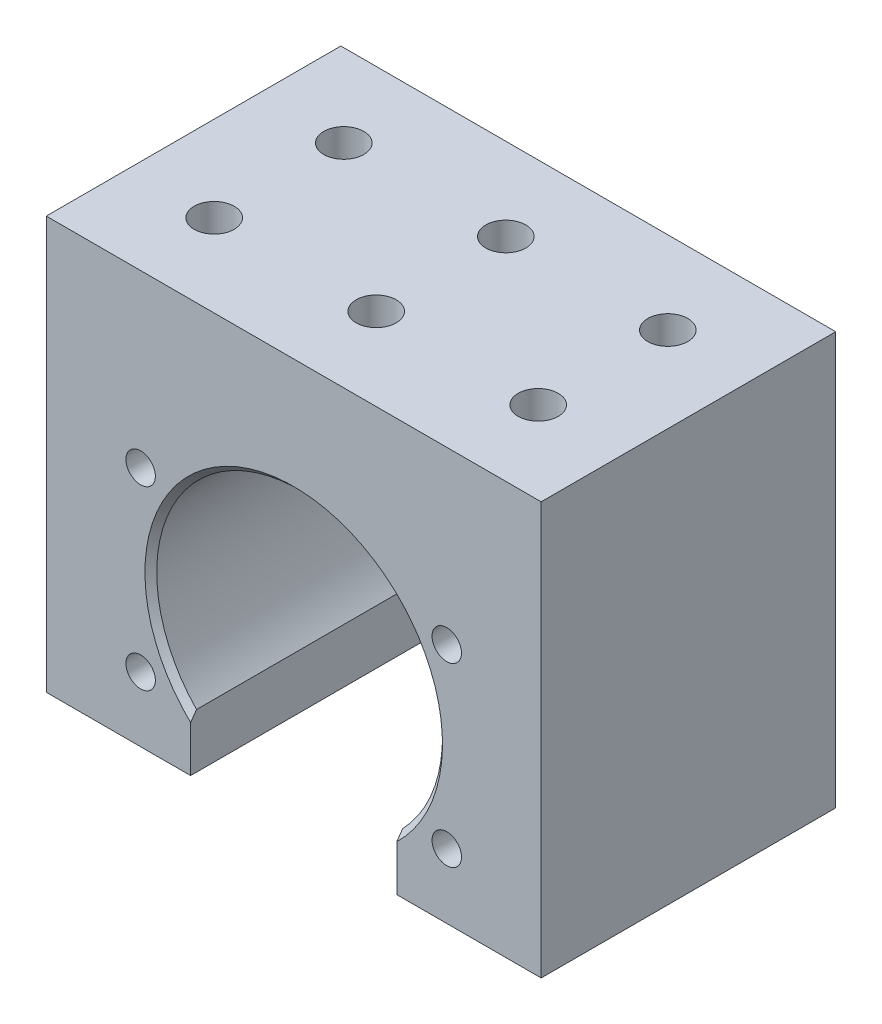
from build123d import *

# Parameters (mm, degrees)
SKETCH_1_W             = 84
SKETCH_1_H             = 70
SKETCH_1_R             = 24.25
EXTRUDE_1_DEPTH        = 25
SKETCH_2_W             = 35
SKETCH_2_H             = 9.212728036
CUT_EXTRUDE_1_DEPTH    = 75.087785768
HOLE_WIZARD_M6_1_D     = 5
HOLE_WIZARD_M8_1_D     = 6.8
HOLE_WIZARD_M8_1_DEPTH = 19.75
HOLE_WIZARD_M8_1_TIP   = 2.042926105
CHAMFER_2_SIZE         = 1


with BuildPart() as part:
    # 草图1 → 凸台-拉伸1 (new, symmetric)
    with BuildSketch(Plane.XY):
        Rectangle(SKETCH_1_W, SKETCH_1_H)
        with Locations((0, -9)):
            Circle(SKETCH_1_R, mode=Mode.SUBTRACT)
    extrude(amount=EXTRUDE_1_DEPTH, both=True)

    # 草图2 → 切除-拉伸1 (cut, through all)
    with BuildSketch(Plane.XY.offset(25)):
        with Locations((0, -30.393635982)):
            Rectangle(SKETCH_2_W, SKETCH_2_H)
    extrude(amount=-CUT_EXTRUDE_1_DEPTH, mode=Mode.SUBTRACT)

    # M6 螺纹孔1 (through all)
    with Locations(Plane(origin=(0, 0, -25), x_dir=(-1, 0, 0), z_dir=(0, 0, -1))):
        with Locations((-25.980762114, 6), (25.980762114, 6), (25.980762114, -24), (-25.980762114, -24)):
            Hole(HOLE_WIZARD_M6_1_D / 2)

    # M8 螺纹孔1
    with Locations(Plane(origin=(0, 35, 0), x_dir=(1, 0, 0), z_dir=(0, 1, 0))):
        with Locations((-27.5, 11), (-27.5, -11), (27.5, -11), (27.5, 11), (0, 11), (0, -11)):
            Hole(HOLE_WIZARD_M8_1_D / 2, depth=HOLE_WIZARD_M8_1_DEPTH)
            with Locations((0, 0, -(HOLE_WIZARD_M8_1_DEPTH + HOLE_WIZARD_M8_1_TIP / 2))):  # 118° drill point
                Cone(0, HOLE_WIZARD_M8_1_D / 2, HOLE_WIZARD_M8_1_TIP, mode=Mode.SUBTRACT)

    # 倒角2
    chamfer_2_edges = [part.edges().sort_by_distance(p)[0] for p in [
        (0, 15.25, 25),
        (0, 15.25, -25),
    ]]
    chamfer(chamfer_2_edges, length=CHAMFER_2_SIZE)


solid = part.part
